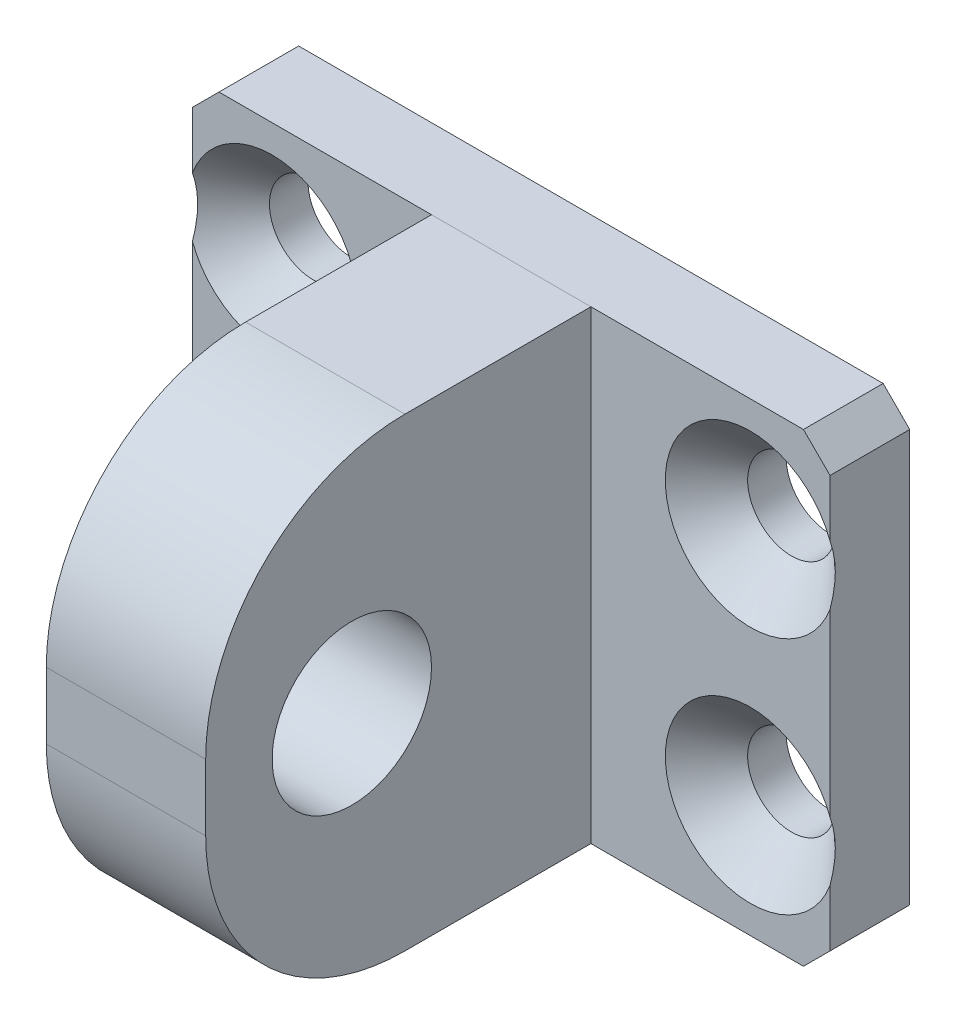
from build123d import *

# Parameters (mm, degrees)
SKETCH1_W                                    = 48
SKETCH1_H                                    = 35
BOSS_EXTRUDE1_DEPTH                          = 6
SKETCH2_W                                    = 12
SKETCH2_H                                    = 35
BOSS_EXTRUDE2_DEPTH                          = 29
FILLET1_R                                    = 15
SKETCH3_R                                    = 6
CUT_EXTRUDE1_DEPTH                           = 20
CHAMFER1_SIZE                                = 2
HOLE_SIZE_SLOTTED_RAISED_COUNTERSUNK_2_COUNT = 2
HOLE_SIZE_SLOTTED_RAISED_COUNTERSUNK_2_PITCH = 18
HOLE_SIZE_SLOTTED_RAISED_COUNTERSUNK_3_COUNT = 2
HOLE_SIZE_SLOTTED_RAISED_COUNTERSUNK_3_PITCH = 36
HOLE_SIZE_SLOTTED_RAISED_COUNTERSUNK_4_COUNT = 2
HOLE_SIZE_SLOTTED_RAISED_COUNTERSUNK_4_PITCH = 40.249223595


with BuildPart() as part:
    # Sketch1 → Boss-Extrude1 (new body)
    with BuildSketch(Plane.XY):
        Rectangle(SKETCH1_W, SKETCH1_H)
    extrude(amount=BOSS_EXTRUDE1_DEPTH)

    # Chamfer1
    chamfer1_edges = [part.edges().sort_by_distance(p)[0] for p in [
        (24, -17.5, 3),
        (-24, -17.5, 3),
        (-24, 17.5, 3),
        (24, 17.5, 3),
    ]]
    chamfer(chamfer1_edges, length=CHAMFER1_SIZE)

    # Sketch5 → Hole Size slotted raised countersunk screw type 1 (revolve, cut)
    with BuildSketch(Plane(origin=(-18, 9, 6), x_dir=(0, -1, 0), z_dir=(1, 0, 0))):
        Polygon((0, 0), (0, 6), (3.3, 6), (3.3, 3.1), (6.4, 0), align=None)
    hole_size_slotted_raised_countersunk_scr = revolve(axis=Axis((-18, 9, 12.35), (0, 0, -1)), mode=Mode.SUBTRACT)

    # Hole Size slotted raised countersunk 2: Hole Size slotted raised countersunk screw type 1 ×2
    with Locations(*[(0, -i * HOLE_SIZE_SLOTTED_RAISED_COUNTERSUNK_2_PITCH, 0) for i in range(1, HOLE_SIZE_SLOTTED_RAISED_COUNTERSUNK_2_COUNT)]):
        add(hole_size_slotted_raised_countersunk_scr, mode=Mode.SUBTRACT)

    # Hole Size slotted raised countersunk 3: Hole Size slotted raised countersunk screw type 1 ×2
    with Locations(*[(i * HOLE_SIZE_SLOTTED_RAISED_COUNTERSUNK_3_PITCH, 0, 0) for i in range(1, HOLE_SIZE_SLOTTED_RAISED_COUNTERSUNK_3_COUNT)]):
        add(hole_size_slotted_raised_countersunk_scr, mode=Mode.SUBTRACT)

    # Hole Size slotted raised countersunk 4: Hole Size slotted raised countersunk screw type 1 ×2
    with Locations(*[Vector(0.894427190999916, -0.447213595499958, 0) * (i * HOLE_SIZE_SLOTTED_RAISED_COUNTERSUNK_4_PITCH) for i in range(1, HOLE_SIZE_SLOTTED_RAISED_COUNTERSUNK_4_COUNT)]):
        add(hole_size_slotted_raised_countersunk_scr, mode=Mode.SUBTRACT)


with BuildPart() as body_2:
    # Sketch2 → Boss-Extrude2 (new body)
    with BuildSketch(Plane.XY.offset(6)):
        Rectangle(SKETCH2_W, SKETCH2_H)
    extrude(amount=BOSS_EXTRUDE2_DEPTH)

    # Fillet1
    fillet1_edges = [body_2.edges().sort_by_distance(p)[0] for p in [
        (0, -17.5, 35),
        (0, 17.5, 35),
    ]]
    fillet(fillet1_edges, radius=FILLET1_R)

    # Sketch3 → Cut-Extrude1 (cut)
    with BuildSketch(Plane(origin=(6, 0, 0), x_dir=(0, 0, -1), z_dir=(1, 0, 0))):
        with Locations((-24, 0)):
            Circle(SKETCH3_R)
    extrude(amount=-CUT_EXTRUDE1_DEPTH, mode=Mode.SUBTRACT)


solid = Compound([part.part, body_2.part])
